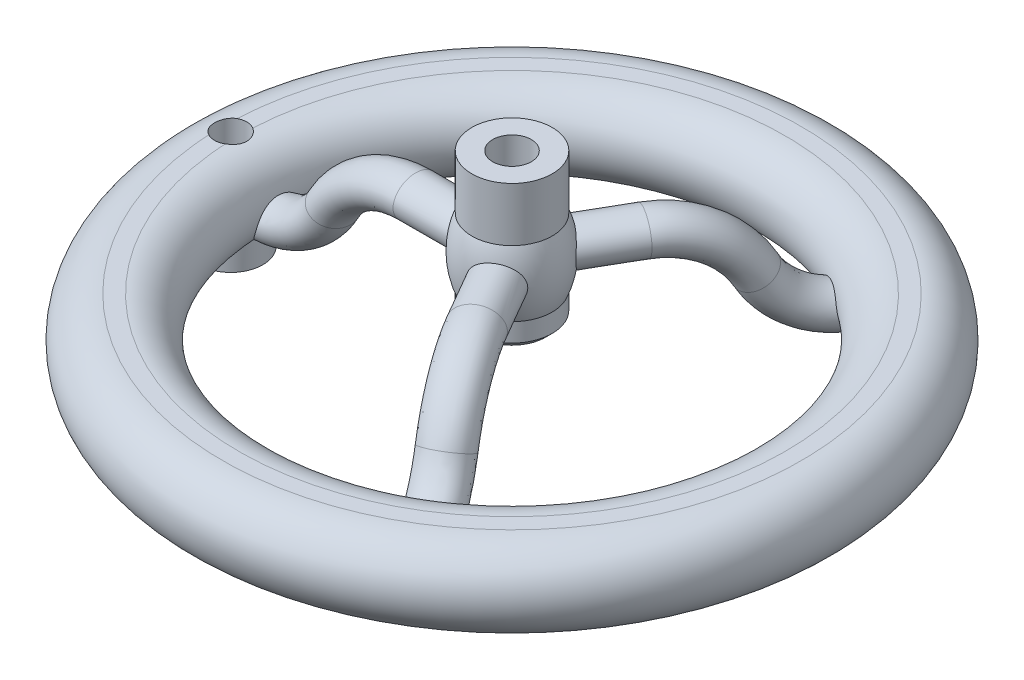
SolidWorks part; units mm, degrees
ref_plane "Front" through (0, 0, 0) normal (0, 0, 1) x (1, 0, 0)
ref_plane "Top" through (0, 0, 0) normal (0, 1, 0) x (1, 0, 0)
ref_plane "Right" through (0, 0, 0) normal (1, 0, 0) x (0, 0, -1)
sketch "Sketch1" plane through (0, 0, 0) normal (0, 0, 1) x (1, 0, 0)
  line L0 (0, 27) -> (0, -18) construction
  line L1 (0, 27) -> (-12.5, 27)
  line L2 (-12.5, 27) -> (-12.5, 10.243)
  line L3 (-12.5, -10.243) -> (-12.5, -16)
  line L4 (-10.5, -18) -> (0, -18)
  line L5 (-12.5, -16) -> (-10.5, -18)
  line L6 (0, 27) -> (0, -18)
  arc A0 (-12.5, 10.243) -> (-12.5, -10.243) centre (12.4816, 0) ccw
  point P6 (-12.5, -18)
  dimension "D1" = 27
  dimension "D2" = 25
  dimension "D3" = 27
  dimension "D4" = 45
  dimension "D5" = 12.4816
revolve "Revolve1" add sketch "Sketch1" angle 360 about L0
sketch "Sketch2" plane through (0, 27, 0) normal (0, 1, 0) x (1, 0, 0)
  circle A0 centre (0, 0) radius 6
  dimension "D1" = 12
extrude "Cut-Extrude1" cut sketch "Sketch2" against normal up to vertex (16.757 mm away) up to point (-12.5, 10.243, 0)
sketch "Sketch3" plane through (0, 0, 0) normal (0, 0, 1) x (1, 0, 0)
  line L0 (0, 0) -> (0, -24) construction
  line L1 (-90, -24) -> (-85, -24) construction
  line L2 (-90, -11.5) -> (-85, -11.5)
  line L3 (-90, -36.5) -> (-85, -36.5)
  arc A0 (-90, -11.5) -> (-90, -36.5) centre (-90, -24) ccw
  arc A1 (-85, -36.5) -> (-85, -11.5) centre (-85, -24) ccw
  point P5 (-87.5, -24)
  dimension "D1" = 12.5
  dimension "D2" = 5
  dimension "D3" = 24
  dimension "D4" = 87.5
revolve "Revolve2" add sketch "Sketch3" angle 360 about L0
sketch "Sketch4" plane through (0, -36.5, 0) normal (0, -1, 0) x (1, 0, 0)
  line L0 (-85, 0) -> (-90, 0) construction
  circle A1 centre (0, 0) radius 85 construction
  circle A2 centre (0, 0) radius 90 construction
  circle A3 centre (-87.5, 0) radius 10
  dimension "D1" = 20
extrude "Boss-Extrude1" add sketch "Sketch4" along normal blind 6 and the other way blind 2
sketch "Sketch5" plane through (0, 0, 0) normal (1, 0, 0) x (0, 0, -1)
  ellipse E0 centre (0, 0) end of major axis (-7, 0) minor radius 6
  dimension "D1" = 12
  dimension "D2" = 14
sketch "Sketch6" plane through (0, 0, 0) normal (0, 0, 1) x (1, 0, 0)
  line L0 (0, 0) -> (-30, 0)
  line L1 (-90, -11.5) -> (-89.4643, -36.5) construction
  arc A0 (-30, 0) -> (-55.5329, -15.2497) centre (-30, -29) ccw
  arc A1 (-55.5329, -15.2497) -> (-89.7321, -24) centre (-76.6636, -3.8701) cw
  dimension "D2" = 29
  dimension "D3" = 24
  dimension "D1" = 30
sweep "Sweep1" add profiles "Sketch5" path "Sketch6"
pattern_circular "CirPattern1" count 3 over 360 of "Sweep1"
sketch "Sketch7" plane through (0, -42.5, 0) normal (0, -1, 0) x (1, 0, 0)
  circle A0 centre (-87.5, 0) radius 5
  dimension "D1" = 10
extrude "Cut-Extrude2" cut sketch "Sketch7" against normal through all
